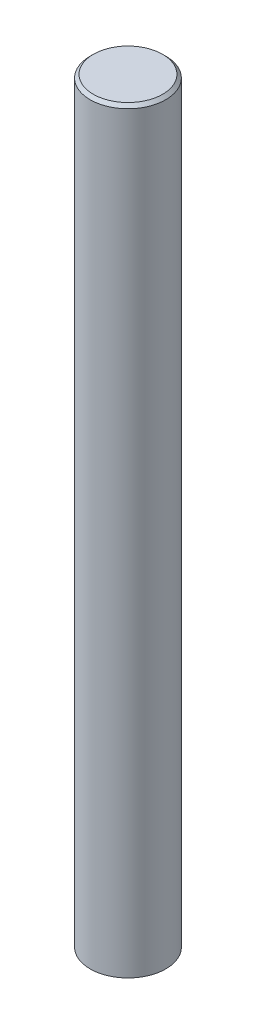
SolidWorks part; units mm, degrees
material "镀铬光轴"
ref_plane "前视" through (0, 0, 0) normal (0, 0, 1) x (1, 0, 0)
ref_plane "上视" through (0, 0, 0) normal (0, 1, 0) x (1, 0, 0)
ref_plane "右视" through (0, 0, 0) normal (1, 0, 0) x (0, 0, -1)
sketch "草图1" plane through (0, 0, 0) normal (0, 1, 0) x (1, 0, 0)
  circle A0 centre (0, 0) radius 6
  dimension "D1" = 12
extrude "凸台-拉伸1" add sketch "草图1" along normal blind 120
sketch "草图2" plane through (0, 0, 0) normal (0, -1, 0) x (1, 0, 0)
  circle A0 centre (0, 0) radius 10
  dimension "D1" = 20
extrude "凸台-拉伸2" [suppressed] add sketch "草图2" against normal blind 6
hole_wizard "M4 螺纹孔1" positions "草图5" profile "草图4" tap size "M4" standard "GB"
sketch "草图5" plane through (0, 0, 0) normal (0, -1, 0) x (-1, 0, 0)
  point P0 (0, 0)
sketch "草图4" plane through (0, 0, 0) normal (1, 0, 0) x (0, 0, -1)
  line L0 (0, 0) -> (0, 16.4914)
  line L1 (0, 16.4914) -> (1.65, 15.5)
  line L2 (1.65, 15.5) -> (1.65, 0)
  line L5 (1.65, 0) -> (0, 0)
  line L10 (0, 16.4914) -> (-1.65, 15.5) construction
  line L11 (0, -6.35) -> (0, 107.95) construction
  dimension "螺纹孔钻头直径" = 3.3
  dimension "螺纹孔钻头深度" = 15.5
  dimension "导头角度" = 118
cosmetic thread "孔螺蚊线1" parameters "D1"=12, "D2"=4
chamfer "倒角1" distance 0.5 angle 45 1 edges at (0, 120, 6)
